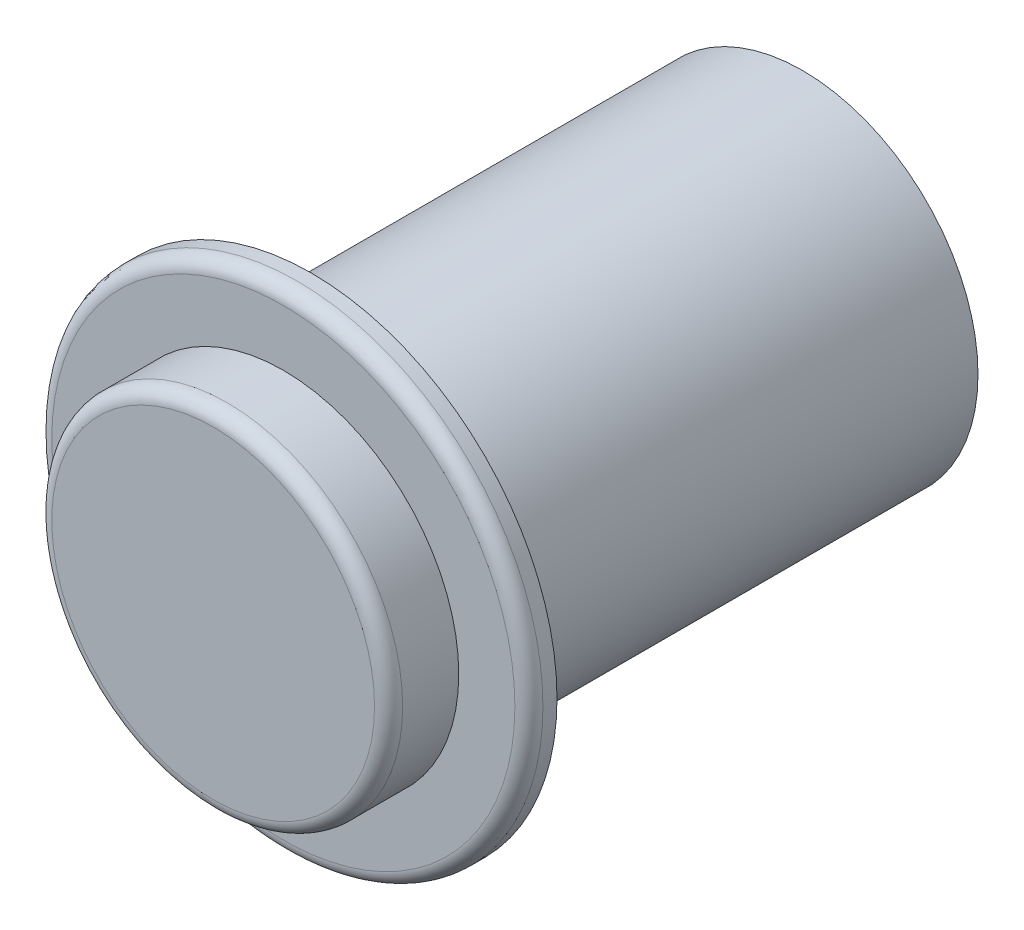
SolidWorks part; units mm, degrees
ref_plane "Front Plane" through (0, 0, 0) normal (0, 0, 1) x (1, 0, 0)
ref_plane "Top Plane" through (0, 0, 0) normal (0, 1, 0) x (1, 0, 0)
ref_plane "Right Plane" through (0, 0, 0) normal (1, 0, 0) x (0, 0, -1)
sketch "Sketch1" plane through (0, 0, 0) normal (0, 0, 1) x (1, 0, 0)
  circle A0 centre (336.1109, 94.2165) radius 12.5 construction
  circle A1 centre (336.1109, 94.2165) radius 12.5
extrude "Boss-Extrude1" add sketch "Sketch1" against normal blind 35
sketch "Sketch2" plane through (0, 0, 0) normal (0, 0, 1) x (1, 0, 0)
  circle A2 centre (336.1109, 94.2165) radius 17.5
  circle A3 centre (336.1109, 94.2165) radius 17.5
  dimension "D1" = 5
extrude "Boss-Extrude2" add sketch "Sketch2" along normal blind 2
sketch "Sketch3" plane through (0, 0, 2) normal (0, 0, 1) x (1, 0, 0)
  circle A2 centre (336.1109, 94.2165) radius 12.5
  circle A3 centre (336.1109, 94.2165) radius 12.5
  dimension "D1" = 5
extrude "Boss-Extrude3" add sketch "Sketch3" along normal blind 5
fillet "Fillet1" radius 1 2 edges at (348.6109, 94.2165, 7) (353.6109, 94.2165, 2)
